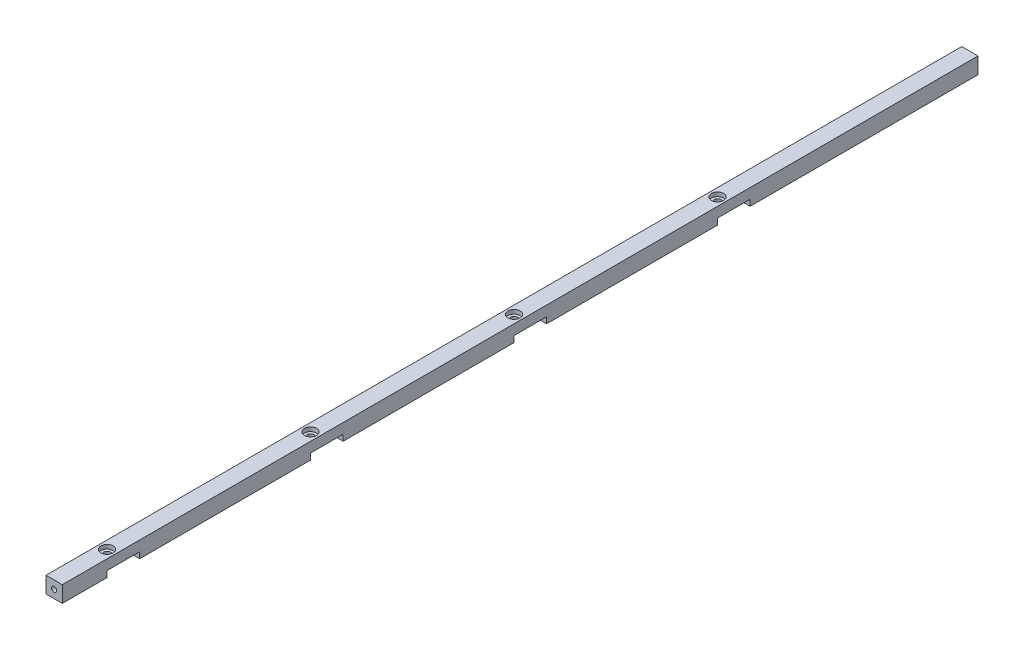
from build123d import *

# Parameters (mm, degrees)
SKETCH_1_W                = 8
SKETCH_1_H                = 8
EXTRUDE_1_DEPTH           = 450
SKETCH_3_W                = 8
SKETCH_3_H                = 16
CUT_EXTRUDE_2_DEPTH       = 3
HOLE_WIZARD_M3_1_D        = 2.5
HOLE_WIZARD_M3_1_DEPTH    = 12
HOLE_WIZARD_M3_1_TIP      = 0.751075774
HOLE_WIZARD_M3_2_D        = 2.5
HOLE_WIZARD_M3_2_DEPTH    = 12
HOLE_WIZARD_M3_2_TIP      = 0.751075774
SKETCH_10_W               = 16
SKETCH_10_H               = 3
CUT_EXTRUDE_3_DEPTH       = 451.088880111
HOLE_WIZARD_1_D           = 3.4
HOLE_WIZARD_1_CBORE_D     = 6
HOLE_WIZARD_1_CBORE_DEPTH = 2


with BuildPart() as part:
    # 草图1 → 凸台-拉伸1 (new body)
    with BuildSketch(Plane.XY):
        Rectangle(SKETCH_1_W, SKETCH_1_H)
    extrude(amount=EXTRUDE_1_DEPTH)

    # 草图3 → 切除-拉伸2 (cut)
    with BuildSketch(Plane.XZ.offset(4)):
        with Locations((0, 420)):
            Rectangle(SKETCH_3_W, SKETCH_3_H)
    extrude(amount=-CUT_EXTRUDE_2_DEPTH, mode=Mode.SUBTRACT)

    # M3 螺纹孔1
    with Locations(Plane(origin=(0, 0, 0), x_dir=(-1, 0, 0), z_dir=(0, 0, -1))):
        with Locations((0, 0)):
            Hole(HOLE_WIZARD_M3_1_D / 2, depth=HOLE_WIZARD_M3_1_DEPTH)
            with Locations((0, 0, -(HOLE_WIZARD_M3_1_DEPTH + HOLE_WIZARD_M3_1_TIP / 2))):  # 118° drill point
                Cone(0, HOLE_WIZARD_M3_1_D / 2, HOLE_WIZARD_M3_1_TIP, mode=Mode.SUBTRACT)

    # M3 螺纹孔2
    with Locations(Plane.XY.offset(450)):
        with Locations((0, 0)):
            Hole(HOLE_WIZARD_M3_2_D / 2, depth=HOLE_WIZARD_M3_2_DEPTH)
            with Locations((0, 0, -(HOLE_WIZARD_M3_2_DEPTH + HOLE_WIZARD_M3_2_TIP / 2))):  # 118° drill point
                Cone(0, HOLE_WIZARD_M3_2_D / 2, HOLE_WIZARD_M3_2_TIP, mode=Mode.SUBTRACT)

    # 草图10 → 切除-拉伸3 (cut, through all)
    with BuildSketch(Plane(origin=(4, 0, 0), x_dir=(0, 0, -1), z_dir=(1, 0, 0))):
        with Locations((-320, -2.5)):
            Rectangle(SKETCH_10_W, SKETCH_10_H)
        with Locations((-220, -2.5)):
            Rectangle(SKETCH_10_W, SKETCH_10_H)
        with Locations((-120, -2.5)):
            Rectangle(SKETCH_10_W, SKETCH_10_H)
    extrude(amount=-CUT_EXTRUDE_3_DEPTH, mode=Mode.SUBTRACT)

    # 打孔尺寸根据内六角圆柱头螺钉的类型1 (through all)
    with Locations(Plane(origin=(0, 4, 0), x_dir=(1, 0, 0), z_dir=(0, 1, 0))):
        with Locations((0, -124), (0, -224), (0, -324), (0, -424)):
            CounterBoreHole(HOLE_WIZARD_1_D / 2, HOLE_WIZARD_1_CBORE_D / 2, HOLE_WIZARD_1_CBORE_DEPTH)


solid = part.part
